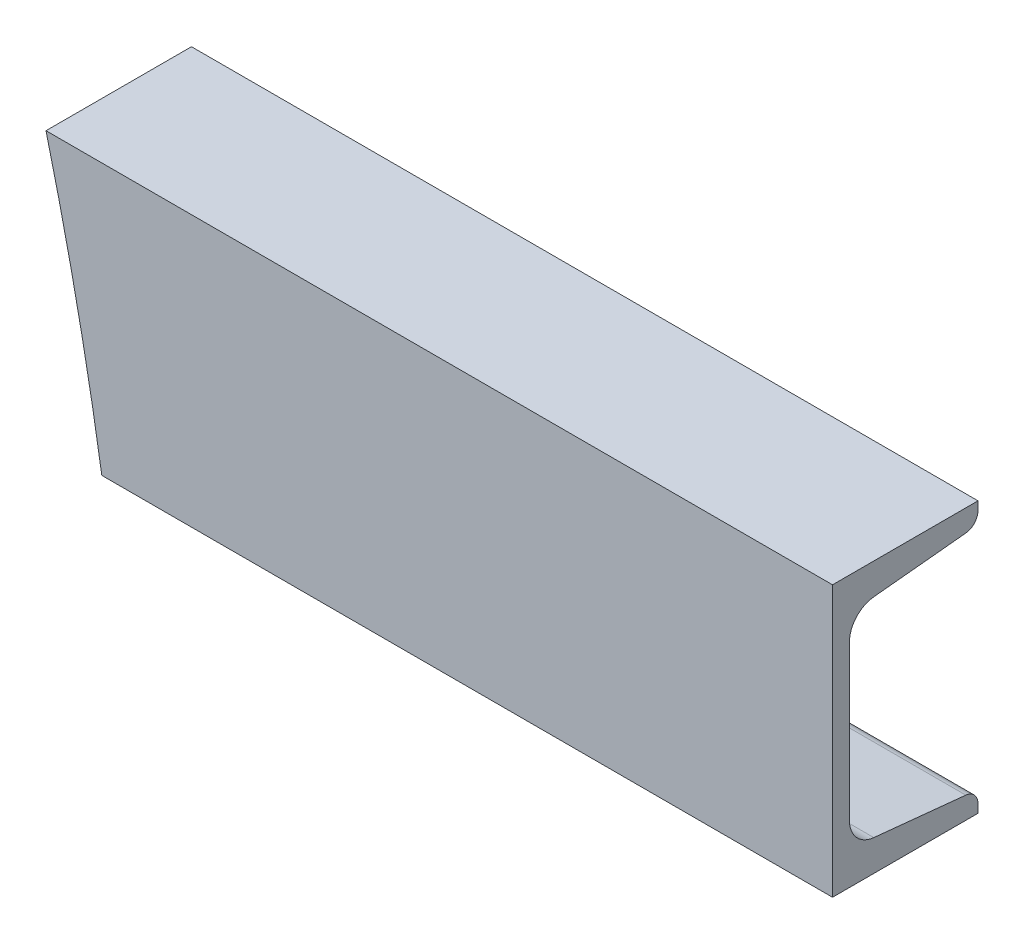
from build123d import *

# Parameters (mm, degrees)
GB_T707_1988_8_XXXXXXXXXXXXXXX528V9_1_DEPTH = 300
CUT_EXTRUDE_2_REACH                         = 315.447
SKETCH_4_R                                  = 895


with BuildPart() as part:
    # Sketch11 → 热轧普通槽钢(gb t707-1988) 8-XXXXXXXXXXXXXXX528V9(1) (new body)
    with BuildSketch(Plane(origin=(0, 0, 0), x_dir=(0, 0, -1), z_dir=(-1, 0, 0))):
        with BuildLine():
            Line((43, 80), (0, 80))
            Line((0, 80), (0, 0))
            Line((0, 0), (43, 0))
            Line((43, 0), (43, 2.480049752))
            ThreePointArc((43, 2.480049752), (41.965810134, 5.164071035), (39.398014876, 6.460198512))
            Line((39.398014876, 6.460198512), (12.203970248, 9.179602975))
            ThreePointArc((12.203970248, 9.179602975), (7.068379732, 11.771857931), (5, 17.139900497))
            Line((5, 17.139900497), (5, 62.860099503))
            ThreePointArc((5, 62.860099503), (7.068379732, 68.228142069), (12.203970248, 70.820397025))
            Line((12.203970248, 70.820397025), (39.398014876, 73.539801488))
            ThreePointArc((39.398014876, 73.539801488), (41.965810134, 74.835928965), (43, 77.519950248))
            Line((43, 77.519950248), (43, 80))
        make_face()
    extrude(amount=-GB_T707_1988_8_XXXXXXXXXXXXXXX528V9_1_DEPTH)

    # 草图4 → 切除-拉伸2 (cut, up to next)
    with BuildSketch(Plane.XY, mode=Mode.PRIVATE) as cut_extrude_2_sk1:
        with Locations((-799.887205022, -220.600173536)):
            Circle(SKETCH_4_R)
    cut_extrude_2_tool1 = extrude(cut_extrude_2_sk1.sketch, amount=-CUT_EXTRUDE_2_REACH, mode=Mode.PRIVATE) & part.part
    add(cut_extrude_2_tool1.solids().sort_by_distance((-799.887205, -220.600174, 0))[0], mode=Mode.SUBTRACT)


solid = part.part
